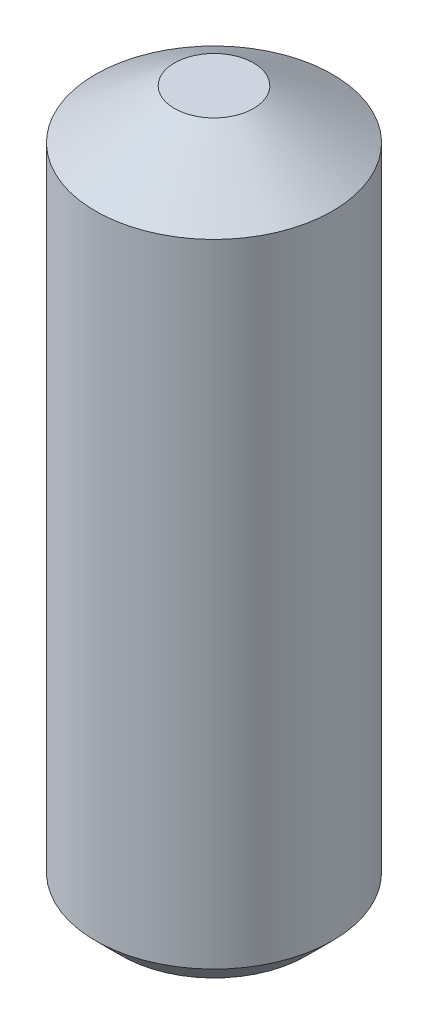
from build123d import *

# Parameters (mm, degrees)
CHAMFER1_SIZE = 1


with BuildPart() as part:
    # Sketch1 → Revolve1 (revolve)
    with BuildSketch(Plane.XY):
        Polygon((0, 26.874718128), (1.5, 26.874718128), (4.500176152, 25), (4.500176152, 0), (0, 0), align=None)
    revolve(axis=Axis((0, 0, 0), (0, 1, 0)))

    # Chamfer1
    chamfer1_edges = [part.edges().sort_by_distance(p)[0] for p in [
        (-4.500176152, 0, 0),
    ]]
    chamfer(chamfer1_edges, length=CHAMFER1_SIZE)


solid = part.part
